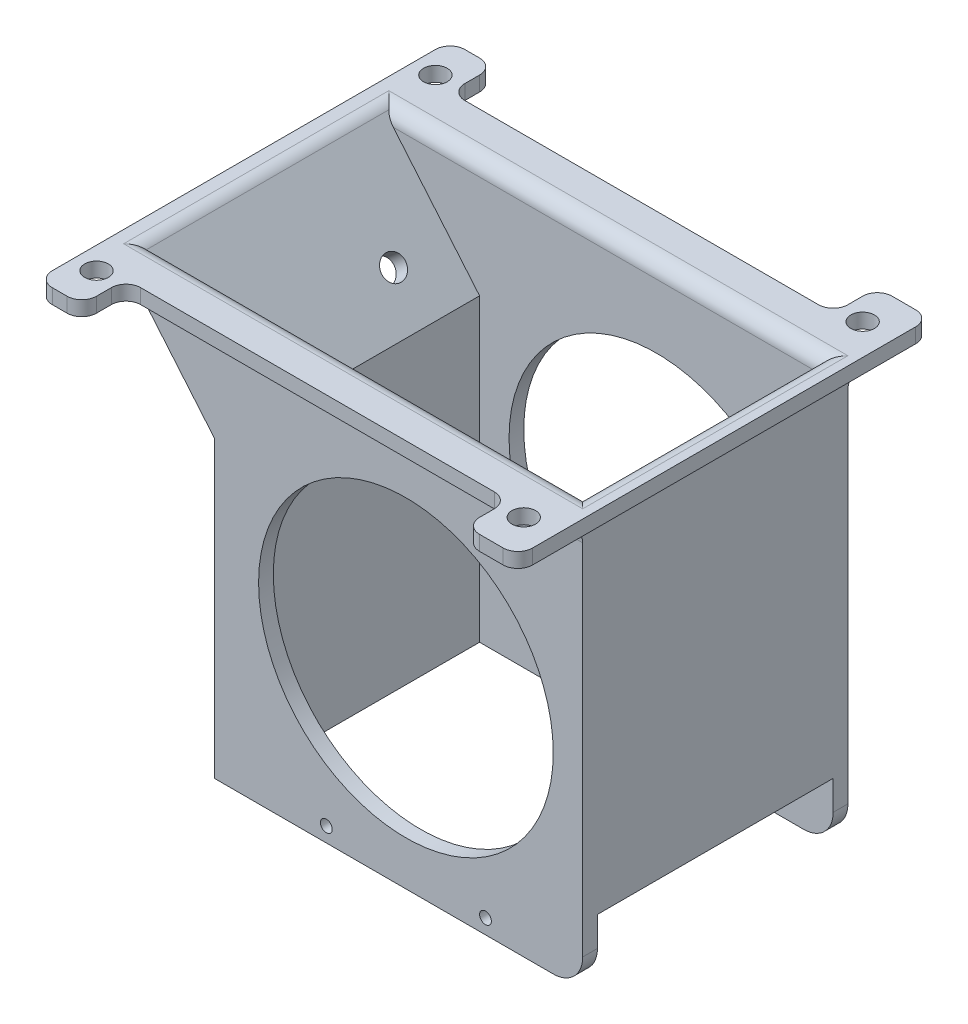
SolidWorks part; units mm, degrees
ref_plane "前视基准面" through (0, 0, 0) normal (0, 0, 1) x (1, 0, 0)
ref_plane "上视基准面" through (0, 0, 0) normal (0, 1, 0) x (1, 0, 0)
ref_plane "右视基准面" through (0, 0, 0) normal (1, 0, 0) x (0, 0, -1)
sketch "草图1" plane through (0, 0, 0) normal (0, 0, 1) x (1, 0, 0)
  line L0 (-65, 0) -> (60, 0)
  line L1 (60, 0) -> (60, 141.7114)
  line L2 (60, 141.7114) -> (-100, 141.7114)
  line L3 (-65, 0) -> (-65, 100)
  line L4 (-65, 100) -> (-100, 141.7114)
  dimension "D1" = 160
  dimension "D2" = 60
  dimension "D3" = 125
  dimension "D4" = 100
  dimension "D5" = 140
extrude "拉伸1" add sketch "草图1" along normal mid plane 90
sketch "草图2" plane through (0, 141.7114, 0) normal (0, 1, 0) x (1, 0, 0)
  line L0 (60, 45) -> (60, 70)
  line L1 (60, 70) -> (45, 70)
  line L2 (45, 70) -> (45, 45)
  line L3 (60, 45) -> (-100, 45) construction
  line L4 (45, 45) -> (60, 45)
  line L6 (-100, 0) -> (95.3242, 0) construction
  line L7 (-100, -45) -> (-100, 45) construction
  line L8 (-20, 45) -> (-20, -62.3483) construction
  line L9 (-100, -45) -> (-100, -70)
  line L10 (-100, -70) -> (-85, -70)
  line L11 (-85, -70) -> (-85, -45)
  line L12 (45, -45) -> (60, -45)
  line L13 (45, -70) -> (45, -45)
  line L14 (60, -70) -> (45, -70)
  line L15 (-85, -45) -> (-100, -45)
  line L16 (-85, 45) -> (-100, 45)
  line L17 (-85, 70) -> (-85, 45)
  line L18 (-100, 70) -> (-85, 70)
  line L19 (60, -45) -> (60, -70)
  line L20 (-100, 45) -> (-100, 70)
  circle A0 centre (52.5, 57.5) radius 4
  circle A1 centre (-92.5, -57.5) radius 4
  circle A2 centre (52.5, -57.5) radius 4
  circle A3 centre (-92.5, 57.5) radius 4
  dimension "D3" = 12.5
  dimension "D4" = 8
  dimension "D5" = 7.5
  dimension "D1" = 25
  dimension "D2" = 15
shell "抽壳1" thickness 5
extrude "拉伸2" add sketch "草图2" against normal blind 5
sketch "草图3" plane through (0, 5, 0) normal (0, 1, 0) x (1, 0, 0)
  line L1 (-60, 40) -> (55, 40)
  line L2 (-60, 40) -> (-60, -40)
  line L3 (-60, -40) -> (55, -40)
  line L4 (55, 40) -> (55, -40)
extrude "拉伸3" cut sketch "草图3" against normal through all
sketch "草图4" plane through (60, 0, 0) normal (1, 0, 0) x (0, 0, -1)
  line L1 (-40, 0) -> (40, 0)
  line L2 (-40, 0) -> (-40, 20)
  line L3 (-40, 20) -> (40, 20)
  line L4 (40, 0) -> (40, 20)
  dimension "D1" = 20
extrude "拉伸4" cut sketch "草图4" against normal blind 5
sketch "草图5" plane through (0, 0, 45) normal (0, 0, 1) x (1, 0, 0)
  line L0 (-65, 0) -> (60, 0) construction
  line L1 (45, 141.7114) -> (-85, 141.7114) construction
  circle A0 centre (0, 65) radius 50
  point P4 (-20, 141.7114)
  dimension "D1" = 100
  dimension "D2" = 65
  dimension "D3" = 20
extrude "拉伸5" cut sketch "草图5" against normal through all
sketch "草图6" plane through (0, 0, 40) normal (0, 0, -1) x (-1, 0, 0)
  line L0 (-55, 102.1643) -> (-46.5794, 88.1163)
  line L1 (-55, 20) -> (-55, 141.7114) construction
  line L2 (-55, 102.1643) -> (-55, 26.8648)
  line L3 (-55, 26.8648) -> (-35.3512, 26.8648)
  arc A0 (-46.5794, 88.1163) -> (-35.3512, 26.8648) centre (0, 65) ccw
  dimension "D1" = 52
extrude "拉伸6" add sketch "草图6" along normal up to next
sketch "草图7" plane through (0, 141.7114, 0) normal (0, 1, 0) x (1, 0, 0)
  line L0 (45, 70) -> (45, 45) construction
  line L1 (-85, 45) -> (45, 45)
  line L2 (-85, 45) -> (-85, 55)
  line L3 (-85, 55) -> (45, 55)
  line L4 (45, 45) -> (45, 55)
  line L6 (-85, -45) -> (45, -45)
  line L7 (-85, -45) -> (-85, -55)
  line L8 (-85, -55) -> (45, -55)
  line L9 (45, -45) -> (45, -55)
  line L15 (60, 70) -> (63, 70)
  line L16 (60, 70) -> (60, -70)
  line L17 (60, -70) -> (63, -70)
  line L18 (63, 70) -> (63, -70)
  dimension "D1" = 10
  dimension "D2" = 10
  dimension "D4" = 3
extrude "拉伸7" add sketch "草图7" against normal blind 5
fillet "圆角1" radius 5 2 edges at (-19.2365, 141.7114, -40) (-19.2365, 141.7114, 40)
fillet "圆角2" radius 5 2 edges at (55, 141.7114, 0) (-93.473, 141.7114, 0)
fillet "圆角3" radius 5 1 edges at (55, 102.1643, 0)
fillet "圆角4" radius 5 12 edges at (45, 139.2114, -55) (45, 139.2114, -70) (63, 139.2114, -70) (63, 139.2114, 70) (45, 139.2114, 55) (45, 139.2114, 70) (-100, 139.2114, -70) (-85, 139.2114, -70) (-85, 139.2114, -55) (-100, 139.2114, 70) (-85, 139.2114, 70) (-85, 139.2114, 55)
fillet "圆角5" radius 5 2 edges
fillet "圆角6" radius 10 2 edges at (60, 0, 42.5) (60, 0, -42.5)
sketch "草图15" plane through (14.927, 12.5253, 0) normal (0.766, 0.6428, 0) x (0.6428, -0.766, 0)
  line L2 (-172.836, -45) -> (-172.836, 45) construction
  circle A0 centre (-132.836, -21.25) radius 4
  circle A1 centre (-132.836, 21.25) radius 4
  dimension "D1" = 40
  dimension "D2" = 40
extrude "拉伸16" cut sketch "草图15" against normal through all
sketch "草图16" plane through (0, 0, 45) normal (0, 0, 1) x (1, 0, 0)
  line L1 (-65, 0) -> (50, 0) construction
  circle A0 centre (-27, 5) radius 2
  circle A1 centre (27, 5) radius 2
  circle A2 centre (0, 65) radius 50 construction
  dimension "D1" = 27
  dimension "D2" = 54
  dimension "D4" = 4
  dimension "D5" = 4
  dimension "D3" = 5
  dimension "D6" = 5
extrude "拉伸17" cut sketch "草图16" against normal through all
